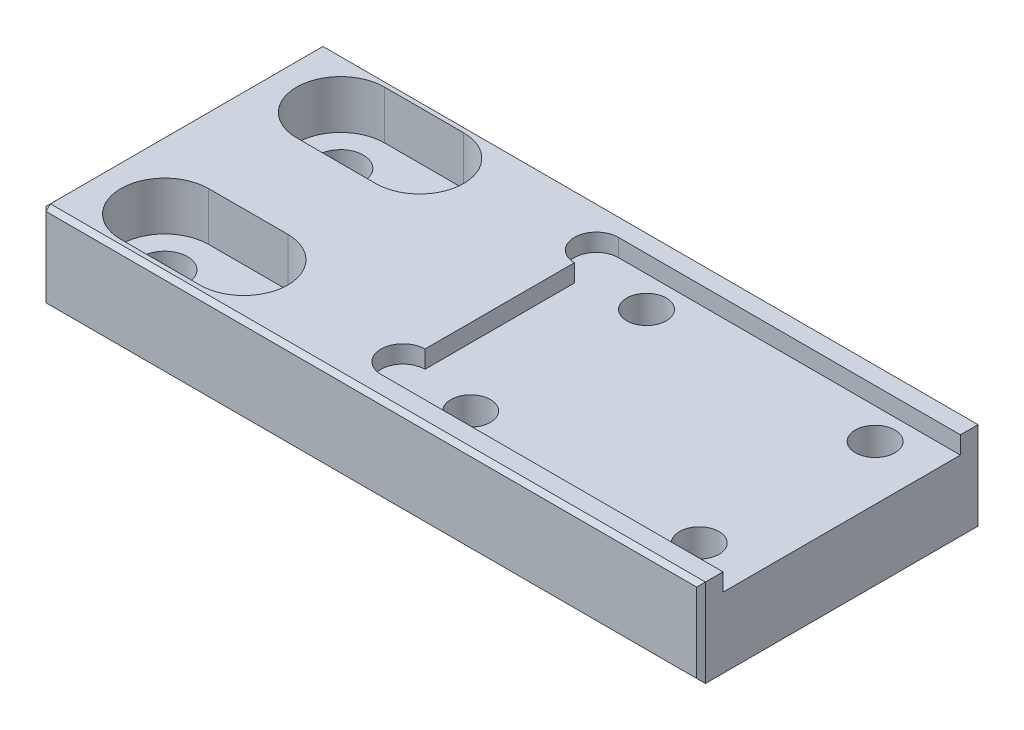
SolidWorks part; units mm, degrees
material "A6061"
ref_plane "前视基准面" through (0, 0, 0) normal (0, 0, 1) x (1, 0, 0)
ref_plane "上视基准面" through (0, 0, 0) normal (0, 1, 0) x (1, 0, 0)
ref_plane "右视基准面" through (0, 0, 0) normal (1, 0, 0) x (0, 0, -1)
sketch "Sketch1" plane through (0, 0, 0) normal (0, 1, 0) x (1, 0, 0)
  line L1 (37.5, -16) -> (-37.5, -16)
  line L2 (37.5, -16) -> (37.5, 16)
  line L3 (37.5, 16) -> (-37.5, 16)
  line L4 (-37.5, -16) -> (-37.5, 16)
  line L5 (37.5, -16) -> (-37.5, 16) construction
  line L6 (37.5, 16) -> (-37.5, -16) construction
  point P0 (0, 0)
  dimension "D1" = 32
  dimension "D2" = 75
extrude "Extrude1" add sketch "Sketch1" along normal blind 10
sketch "Sketch2" plane through (0, 10, 0) normal (0, 1, 0) x (1, 0, 0)
  line L0 (37.5, -16) -> (37.5, 16) construction
  line L1 (37.5, 13.5) -> (-1.4, 13.5)
  line L2 (37.5, 13.5) -> (37.5, -13.5)
  line L3 (37.5, -13.5) -> (-1.4, -13.5)
  line L4 (-1.4, 13.5) -> (-1.4, -13.5)
  line L5 (-37.5, 0) -> (-1.4, 0) construction
  line L6 (-37.5, 16) -> (-37.5, -16) construction
  point P12 (-1.4, -13.5)
  dimension "D1" = 27
  dimension "D2" = 38.9
extrude "Extrude2" cut sketch "Sketch2" against normal blind 2
hole_wizard "CBORE for M4 Hexagon socket head cap screws1" positions "Sketch6" profile "Sketch5" counterbore size "M4" standard "GB" end condition through all
sketch "Sketch6" plane through (0, 0, 0) normal (0, -1, 0) x (-1, 0, 0)
  line L0 (-31.3, 10) -> (-5.3, 10) construction
  line L1 (-5.3, 10) -> (-5.3, -10) construction
  line L2 (-5.3, -10) -> (-31.3, -10) construction
  line L3 (-31.3, -10) -> (-31.3, 10) construction
  line L5 (-37.5, 0) -> (-31.3, 0) construction
  line L6 (-37.5, -16) -> (-37.5, 16) construction
  point P0 (-31.3, -10)
  point P3 (-31.3, 10)
  point P6 (-5.3, 10)
  point P9 (-5.3, -10)
  dimension "D1" = 26
  dimension "D2" = 20
  dimension "D3" = 6.2
sketch "Sketch5" plane through (31.3, 0, 10) normal (1, 0, 0) x (0, 0, -1)
  line L0 (0, 0) -> (0, 10)
  line L1 (0, 10) -> (2.25, 10)
  line L3 (2.25, 10) -> (2.25, 4.6)
  line L4 (2.25, 4.6) -> (4, 4.6)
  line L5 (4, 4.6) -> (4, 0)
  line L7 (4, 0) -> (0, 0)
  line L11 (0, -6.35) -> (0, 107.95) construction
  dimension "通孔孔直径" = 4.5
  dimension "通孔孔深度" = 10
  dimension "柱形沉头孔直径" = 8
  dimension "柱形沉头孔深度" = 4.6
hole_wizard "CBORE for M5 Hexagon socket head cap screws1" positions "Sketch9" profile "Sketch8" counterbore size "M5" standard "GB" end condition through all
sketch "Sketch9" plane through (0, 10, 0) normal (0, 1, 0) x (1, 0, 0)
  line L0 (-29.5, 10) -> (-29.5, -10) construction
  line L1 (-29.5, -10) -> (-20.5, -10) construction
  line L2 (-20.5, -10) -> (-20.5, 10) construction
  line L3 (-20.5, 10) -> (-29.5, 10) construction
  line L5 (-37.5, 0) -> (-29.5, 0) construction
  line L6 (-37.5, 16) -> (-37.5, -16) construction
  point P0 (-29.5, 10)
  point P2 (-20.5, 10)
  point P4 (-20.5, -10)
  point P6 (-29.5, -10)
  dimension "D1" = 8
  dimension "D2" = 20
  dimension "D3" = 9
sketch "Sketch8" plane through (-29.5, 10, -10) normal (1, 0, 0) x (0, 0, 1)
  line L0 (0, 0) -> (0, 10)
  line L1 (0, 10) -> (2.6, 10)
  line L3 (2.6, 10) -> (2.6, 5.5)
  line L4 (2.6, 5.5) -> (5, 5.5)
  line L5 (5, 5.5) -> (5, 0)
  line L7 (5, 0) -> (0, 0)
  line L11 (0, -6.35) -> (0, 107.95) construction
  dimension "通孔孔直径" = 5.2
  dimension "通孔孔深度" = 10
  dimension "柱形沉头孔直径" = 10
  dimension "柱形沉头孔深度" = 5.5
sketch "Sketch10" plane through (0, 4.5, 0) normal (0, 1, 0) x (1, 0, 0)
  line L0 (-29.5, 10) -> (-20.5, 10) construction
  line L1 (-29.5, 15) -> (-20.5, 15)
  line L2 (-29.5, 5) -> (-20.5, 5)
  line L3 (-29.5, -10) -> (-20.5, -10) construction
  line L4 (-29.5, -5) -> (-20.5, -5)
  line L5 (-29.5, -15) -> (-20.5, -15)
  arc A0 (-29.5, 15) -> (-29.5, 5) centre (-29.5, 10) ccw
  arc A1 (-20.5, 5) -> (-20.5, 15) centre (-20.5, 10) ccw
  arc A2 (-29.5, -5) -> (-29.5, -15) centre (-29.5, -10) ccw
  arc A3 (-20.5, -15) -> (-20.5, -5) centre (-20.5, -10) ccw
  point P2 (-25, 10)
  point P9 (-25, -10)
  dimension "D1" = 5
extrude "Extrude4" cut sketch "Sketch10" along normal blind 10
sketch "Sketch11" plane through (0, 10, 0) normal (0, 1, 0) x (1, 0, 0)
  line L0 (-1.4, 13.5) -> (-1.4, -13.5) construction
  circle A0 centre (-1.4, 11) radius 2.5
  circle A1 centre (-1.4, -11) radius 2.5
  dimension "D1" = 5
extrude "Extrude6" cut sketch "Sketch11" against normal up to surface (2 mm away) up to face at (31.3, 8, 7.75)
chamfer "Chamfer1" distance 0.5 angle 45 9 edges at (0, 10, 16) (0, 10, -16) (37.5, 5, -16) (0, 0, -16) (-37.5, 5, -16) (-37.5, 10, 0) (-37.5, 5, 16) (0, 0, 16) (37.5, 5, 16)
